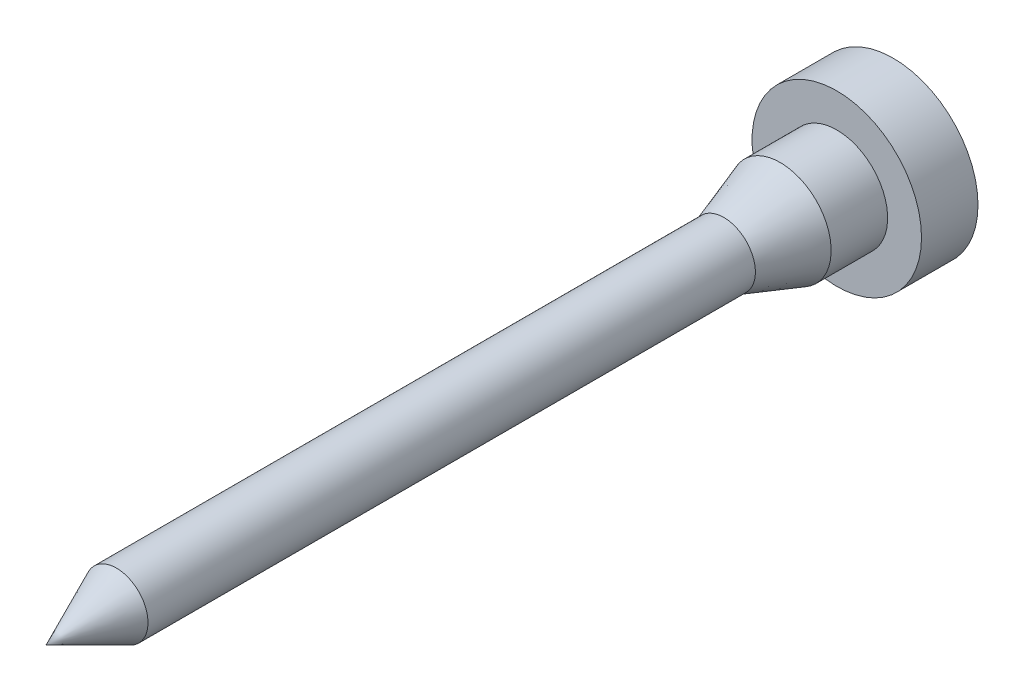
SolidWorks part; units mm, degrees
ref_plane "Front Plane" through (0, 0, 0) normal (0, 0, 1) x (1, 0, 0)
ref_plane "Top Plane" through (0, 0, 0) normal (0, 1, 0) x (1, 0, 0)
ref_plane "Right Plane" through (0, 0, 0) normal (1, 0, 0) x (0, 0, -1)
sketch "Sketch1" plane through (0, 0, 0) normal (0, 0, 1) x (1, 0, 0)
  circle A0 centre (0, 0) radius 15
  dimension "D1" = 30
extrude "Boss-Extrude1" add sketch "Sketch1" along normal blind 10
sketch "Sketch2" plane through (0, 0, 0) normal (0, 1, 0) x (1, 0, 0)
  line L0 (0, 14.2296) -> (0, -150) construction
  line L1 (9, -10) -> (9, -20)
  line L2 (-15, -10) -> (15, -10) construction
  line L3 (9, -20) -> (5.5859, -30)
  line L4 (5.5859, -30) -> (5.5859, -137.5268)
  line L5 (5.5859, -137.5268) -> (0, -150)
  line L6 (9, -10) -> (0, -10)
  line L7 (0, -10) -> (0, -150)
  dimension "D1" = 140
  dimension "D2" = 9
  dimension "D3" = 10
  dimension "D4" = 10
revolve "Revolve1" add sketch "Sketch2" angle 360 about L0
